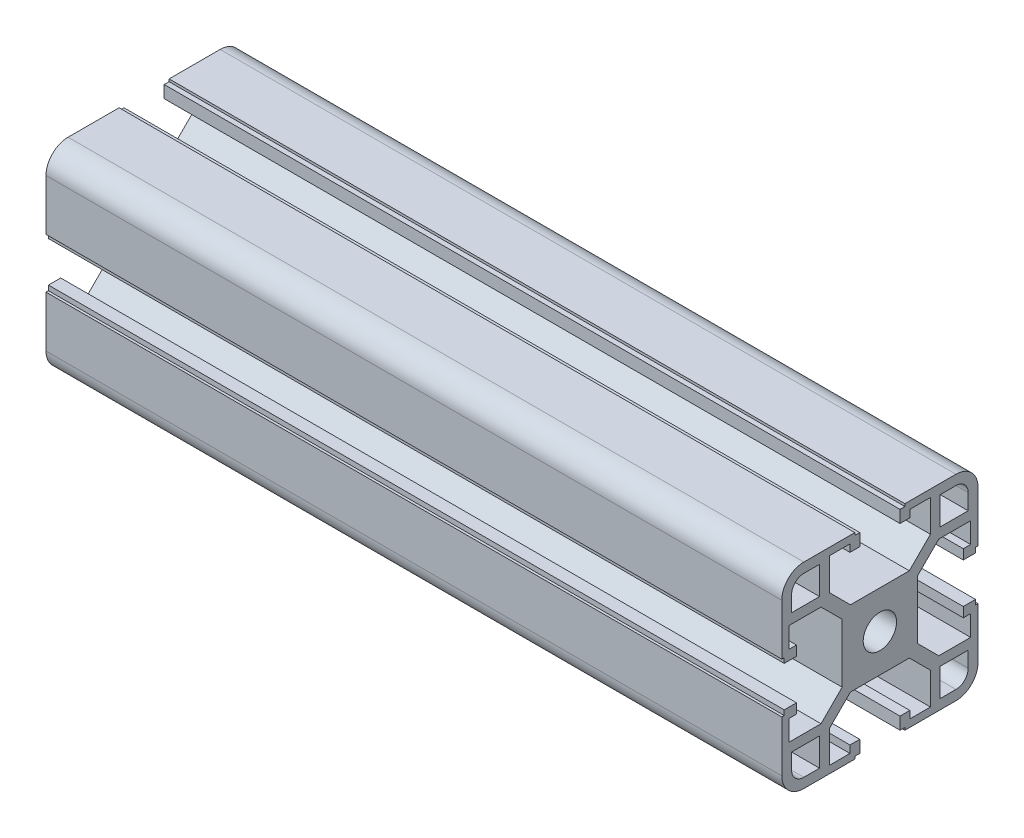
SolidWorks part; units mm, degrees
ref_plane "Front Plane" through (0, 0, 0) normal (0, 0, 1) x (1, 0, 0)
ref_plane "Top Plane" through (0, 0, 0) normal (0, 1, 0) x (1, 0, 0)
ref_plane "Right Plane" through (0, 0, 0) normal (1, 0, 0) x (0, 0, -1)
sketch "草图1" plane through (0, 0, 0) normal (0, 0, 1) x (1, 0, 0)
  line L0 (0, 0) -> (150, 0)
  dimension "D1" = 150
other "Aluminum profile 40 X 40B X R4.5(1)"
ref_plane "Plane1" through (0, 0, 0) normal (1, 0, 0) x (0, 1, 0)
sketch "Sketch1" plane through (0, 0, 0) normal (1, 0, 0) x (0, 1, 0)
  line L0 (-5.1, 20) -> (-5.1, 19.5)
  line L1 (-5.1, 19.5) -> (-4.1, 19.5)
  line L2 (-4.1, 19.5) -> (-4.1, 17)
  line L3 (-6.1, 18.5) -> (-10.3, 18.5)
  line L4 (-15.5, -20) -> (-5.1, -20)
  line L5 (-20, -15.5) -> (-20, -5.1)
  line L6 (15.5, 20) -> (5.1, 20)
  line L7 (20, 15.5) -> (20, 5.1)
  line L8 (0, 14.8756) -> (0, 0) construction
  line L9 (0, 0) -> (14.1675, 0) construction
  line L10 (-10.3, 18.5) -> (-10.3, 12)
  line L11 (-10.3, 12) -> (-6, 7.7)
  line L12 (-6, 7.7) -> (6, 7.7)
  line L13 (10.3, 12) -> (6, 7.7)
  line L14 (10.3, 18.5) -> (10.3, 12)
  line L15 (6.1, 18.5) -> (10.3, 18.5)
  line L16 (4.1, 19.5) -> (4.1, 17)
  line L17 (5.1, 19.5) -> (4.1, 19.5)
  line L18 (5.1, 20) -> (5.1, 19.5)
  line L19 (-5.1, 20) -> (-15.5, 20)
  line L20 (20, 5.1) -> (19.5, 5.1)
  line L21 (12.3, 18) -> (15.5, 18)
  line L22 (12.3, 18) -> (12.3, 12.3)
  line L23 (12.3, 12.3) -> (18, 12.3)
  line L24 (18, 15.5) -> (18, 12.3)
  line L25 (19.5, 5.1) -> (19.5, 4.1)
  line L26 (19.5, 4.1) -> (17, 4.1)
  line L27 (17, 6.1) -> (17, 4.1)
  line L28 (18.5, 6.1) -> (17, 6.1)
  line L29 (18.5, 6.1) -> (18.5, 10.3)
  line L30 (18.5, 10.3) -> (12, 10.3)
  line L31 (12, 10.3) -> (7.7, 6)
  line L32 (7.7, 6) -> (7.7, -6)
  line L33 (12, -10.3) -> (7.7, -6)
  line L34 (18.5, -10.3) -> (12, -10.3)
  line L35 (18.5, -6.1) -> (18.5, -10.3)
  line L36 (18.5, -6.1) -> (17, -6.1)
  line L37 (17, -4.1) -> (17, -6.1)
  line L38 (19.5, -4.1) -> (17, -4.1)
  line L39 (19.5, -5.1) -> (19.5, -4.1)
  line L40 (20, -5.1) -> (19.5, -5.1)
  line L41 (5.1, -20) -> (5.1, -19.5)
  line L42 (5.1, -19.5) -> (4.1, -19.5)
  line L43 (4.1, -19.5) -> (4.1, -17)
  line L44 (6.1, -17) -> (4.1, -17)
  line L45 (6.1, -18.5) -> (6.1, -17)
  line L46 (6.1, -18.5) -> (10.3, -18.5)
  line L47 (10.3, -18.5) -> (10.3, -12)
  line L48 (10.3, -12) -> (6, -7.7)
  line L49 (6, -7.7) -> (-6, -7.7)
  line L50 (-10.3, -12) -> (-6, -7.7)
  line L51 (-10.3, -18.5) -> (-10.3, -12)
  line L52 (-6.1, -18.5) -> (-10.3, -18.5)
  line L53 (-6.1, -18.5) -> (-6.1, -17)
  line L54 (-4.1, -17) -> (-6.1, -17)
  line L55 (-4.1, -19.5) -> (-4.1, -17)
  line L56 (-5.1, -19.5) -> (-4.1, -19.5)
  line L57 (-5.1, -20) -> (-5.1, -19.5)
  line L58 (-20, -5.1) -> (-19.5, -5.1)
  line L59 (5.1, -20) -> (15.5, -20)
  line L60 (-20, 5.1) -> (-20, 15.5)
  line L61 (-19.5, -5.1) -> (-19.5, -4.1)
  line L62 (-6.1, 18.5) -> (-6.1, 17)
  line L63 (-6.1, 17) -> (-4.1, 17)
  line L64 (6.1, 18.5) -> (6.1, 17)
  line L65 (4.1, 17) -> (6.1, 17)
  line L66 (-19.5, -4.1) -> (-17, -4.1)
  line L67 (-15.5, 18) -> (-12.3, 18)
  line L68 (-18, 15.5) -> (-18, 12.3)
  line L69 (-18, 12.3) -> (-12.3, 12.3)
  line L70 (-12.3, 18) -> (-12.3, 12.3)
  line L71 (-17, -6.1) -> (-17, -4.1)
  line L72 (-18.5, -6.1) -> (-17, -6.1)
  line L73 (-18.5, -6.1) -> (-18.5, -10.3)
  line L74 (-18.5, -10.3) -> (-12, -10.3)
  line L75 (-12, -10.3) -> (-7.7, -6)
  line L76 (-7.7, -6) -> (-7.7, 6)
  line L77 (-12, 10.3) -> (-7.7, 6)
  line L78 (-18.5, 10.3) -> (-12, 10.3)
  line L79 (-18.5, 6.1) -> (-18.5, 10.3)
  line L80 (-18.5, 6.1) -> (-17, 6.1)
  line L81 (-17, 4.1) -> (-17, 6.1)
  line L82 (-19.5, 4.1) -> (-17, 4.1)
  line L83 (-19.5, 5.1) -> (-19.5, 4.1)
  line L84 (-20, 5.1) -> (-19.5, 5.1)
  line L85 (20, -5.1) -> (20, -15.5)
  line L87 (-18, -12.3) -> (-12.3, -12.3)
  line L88 (-18, -12.3) -> (-18, -15.5)
  line L89 (-15.5, -18) -> (-12.3, -18)
  line L90 (-12.3, -12.3) -> (-12.3, -18)
  line L91 (12.3, -12.3) -> (18, -12.3)
  line L92 (12.3, -12.3) -> (12.3, -18)
  line L93 (12.3, -18) -> (15.5, -18)
  line L94 (18, -12.3) -> (18, -15.5)
  circle A0 centre (0, 0) radius 3.4
  arc A1 (-20, 15.5) -> (-15.5, 20) centre (-15.5, 15.5) cw
  arc A2 (20, 15.5) -> (15.5, 20) centre (15.5, 15.5) ccw
  arc A3 (-15.5, -20) -> (-20, -15.5) centre (-15.5, -15.5) cw
  arc A4 (15.5, -20) -> (20, -15.5) centre (15.5, -15.5) ccw
  arc A5 (-15.5, 18) -> (-18, 15.5) centre (-15.5, 15.5) ccw
  arc A6 (18, 15.5) -> (15.5, 18) centre (15.5, 15.5) ccw
  arc A7 (18, -15.5) -> (15.5, -18) centre (15.5, -15.5) cw
  arc A8 (-18, -15.5) -> (-15.5, -18) centre (-15.5, -15.5) ccw
  point P2 (0, 10)
  point P4 (0, 0)
  point P5 (-20, -20)
  point P6 (20, -20)
  point P7 (20, 20)
  point P8 (-20, 20)
  point P36 (-20, 20)
  point P39 (20, 20)
  point P121 (0, 0)
  dimension "D1" = 20.6
  dimension "D2" = 40
  dimension "D3" = 8.2
  dimension "D4" = 10.2
  dimension "D5" = 12.3
  dimension "D6" = 6.8
  dimension "D7" = 4.5
  dimension "D8" = 45
  dimension "D12" = 2
  dimension "D13" = 5.7
  dimension "D14" = 2
  dimension "D18" = 2.5
  dimension "D19" = 2.5
  dimension "D15" = 2.5
  dimension "D9" = 0.5
  dimension "D10" = 1.5
  dimension "D11" = 12
  dimension "D16" = 3
  dimension "D17" = 2
  dimension "D20" = 2
  dimension "D21" = 2
